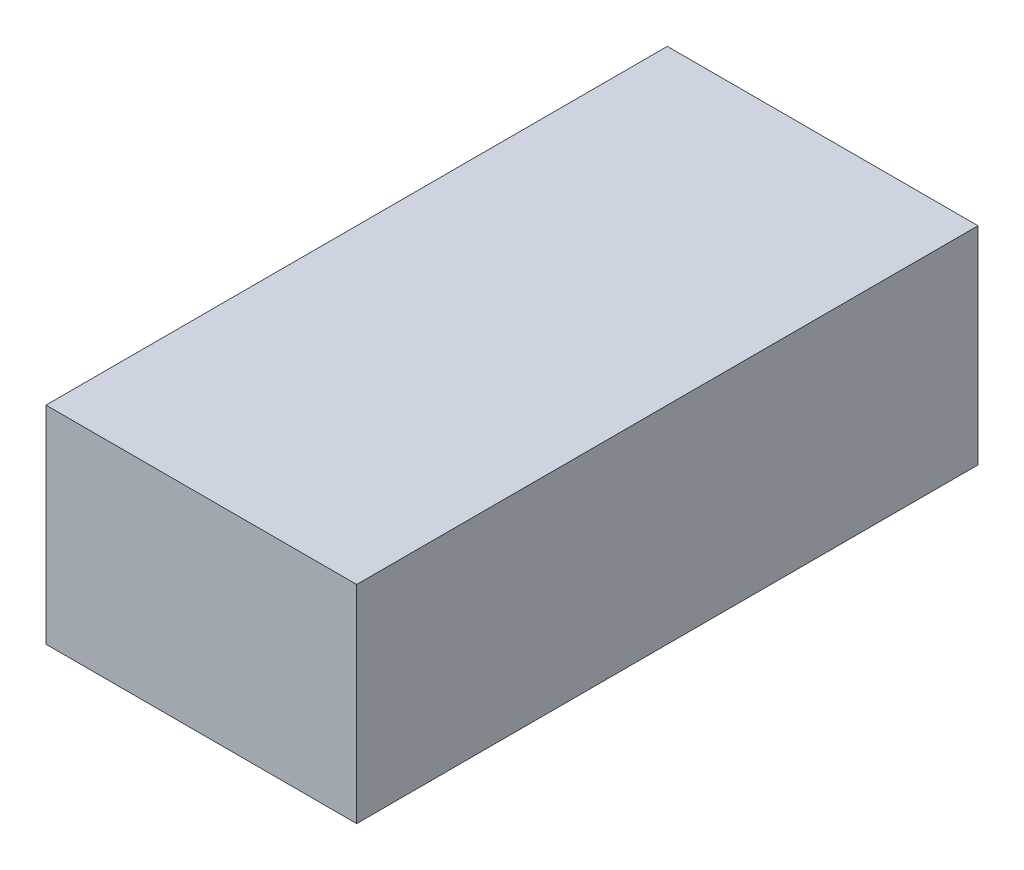
SolidWorks part; units mm, degrees
ref_plane "Front Plane" through (0, 0, 0) normal (0, 0, 1) x (1, 0, 0)
ref_plane "Top Plane" through (0, 0, 0) normal (0, 1, 0) x (1, 0, 0)
ref_plane "Right Plane" through (0, 0, 0) normal (1, 0, 0) x (0, 0, -1)
sketch "Sketch1" plane through (0, 0, 0) normal (0, 0, 1) x (1, 0, 0)
  line L1 (-75, 50) -> (75, 50)
  line L2 (-75, 50) -> (-75, -50)
  line L3 (-75, -50) -> (75, -50)
  line L4 (75, 50) -> (75, -50)
  line L5 (-75, 50) -> (75, -50) construction
  line L6 (-75, -50) -> (75, 50) construction
  point P0 (0, 0)
  dimension "D1" = 150
  dimension "D2" = 100
extrude "Boss-Extrude1" add sketch "Sketch1" along normal blind 300
